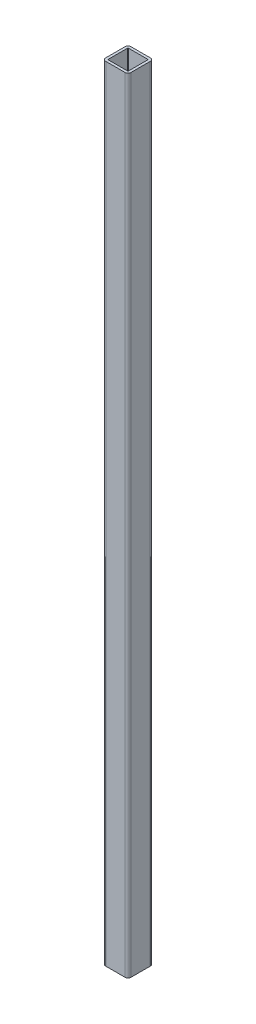
from build123d import *

# Parameters (mm, degrees)
EXTRUDE_1_DEPTH = 1550


with BuildPart() as part:
    # 草图1 → 凸台-拉伸1 (new body)
    with BuildSketch(Plane(origin=(0, 0, 0), x_dir=(1, 0, 0), z_dir=(0, 1, 0))):
        with BuildLine():
            Line((-19, -25), (19, -25))
            ThreePointArc((19, -25), (23.242640687, -23.242640687), (25, -19))
            Line((25, -19), (25, 19))
            ThreePointArc((25, 19), (23.242640687, 23.242640687), (19, 25))
            Line((19, 25), (-19, 25))
            ThreePointArc((-19, 25), (-23.242640687, 23.242640687), (-25, 19))
            Line((-25, 19), (-25, -19))
            ThreePointArc((-25, -19), (-23.242640687, -23.242640687), (-19, -25))
        make_face()
        with BuildLine():
            Line((-19, -20), (19, -20))
            ThreePointArc((19, -20), (19.707106781, -19.707106781), (20, -19))
            Line((20, -19), (20, 19))
            ThreePointArc((20, 19), (19.707106781, 19.707106781), (19, 20))
            Line((19, 20), (-19, 20))
            ThreePointArc((-19, 20), (-19.707106781, 19.707106781), (-20, 19))
            Line((-20, 19), (-20, -19))
            ThreePointArc((-20, -19), (-19.707106781, -19.707106781), (-19, -20))
        make_face(mode=Mode.SUBTRACT)
    extrude(amount=EXTRUDE_1_DEPTH)


solid = part.part
